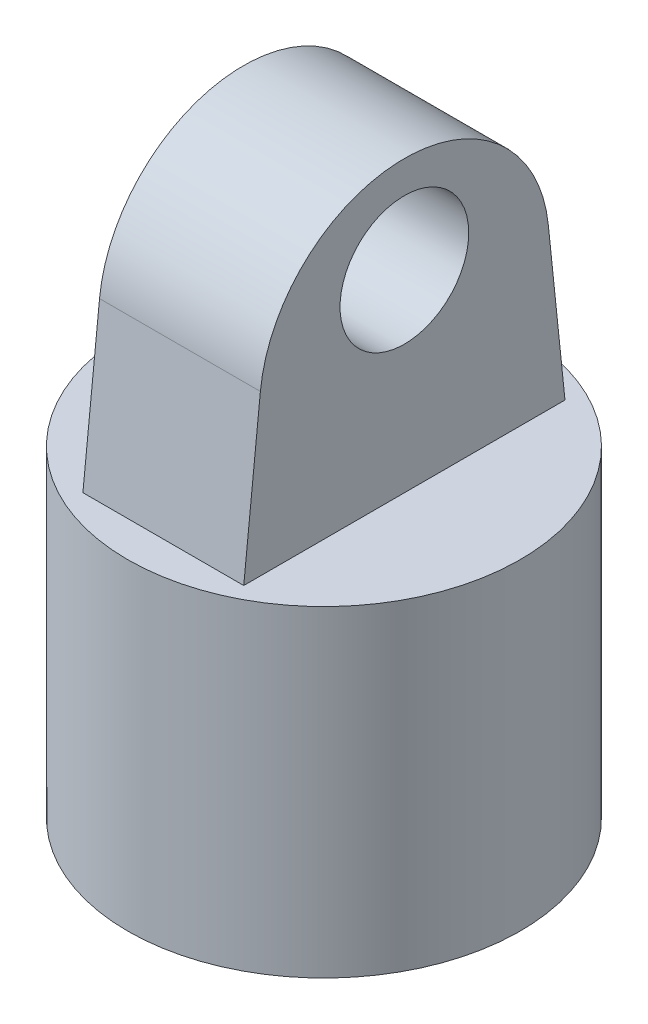
SolidWorks part; units mm, degrees
ref_plane "Front Plane" through (0, 0, 0) normal (0, 0, 1) x (1, 0, 0)
ref_plane "Top Plane" through (0, 0, 0) normal (0, 1, 0) x (1, 0, 0)
ref_plane "Right Plane" through (0, 0, 0) normal (1, 0, 0) x (0, 0, -1)
other "Configuration Table"
sketch "Sketch1" plane through (0, 0, 0) normal (0, 1, 0) x (1, 0, 0)
  circle A0 centre (0, 0) radius 6.1
  dimension "D1" = 12.2
extrude "Boss-Extrude1" add sketch "Sketch1" along normal blind 10
sketch "Sketch2" plane through (0, 0, 0) normal (1, 0, 0) x (0, 0, -1)
  line L0 (0, 0) -> (0, 17.511) construction
  line L1 (-4.9927, 10) -> (-4.4758, 14.9658)
  line L4 (6.1, 10) -> (-6.1, 10) construction
  line L5 (4.9927, 10) -> (4.4758, 14.9658)
  line L6 (-4.9927, 10) -> (4.9927, 10)
  arc A0 (-4.4758, 14.9658) -> (4.4758, 14.9658) centre (0, 14.5) cw
  point P10 (0, 19)
  dimension "D1" = 4.5
  dimension "D2" = 9
extrude "Boss-Extrude2" add sketch "Sketch2" along normal mid plane 5
sketch "Sketch3" plane through (2.5, 0, 0) normal (1, 0, 0) x (0, 0, -1)
  line L1 (6.1, 10) -> (-6.1, 10) construction
  circle A0 centre (0, 16) radius 2
  dimension "D1" = 4
  dimension "D2" = 6
extrude "Cut-Extrude1" cut sketch "Sketch3" against normal through all
sketch "Sketch4" plane through (0, 0, 0) normal (0, -1, 0) x (1, 0, 0)
  circle A0 centre (0, 0) radius 5.6
  dimension "D1" = 11.2
extrude "Cut-Extrude2" cut sketch "Sketch4" against normal blind 5
chamfer "Chamfer1" distance 0.72 angle 45 1 edges at (0, 5, -5.6)
